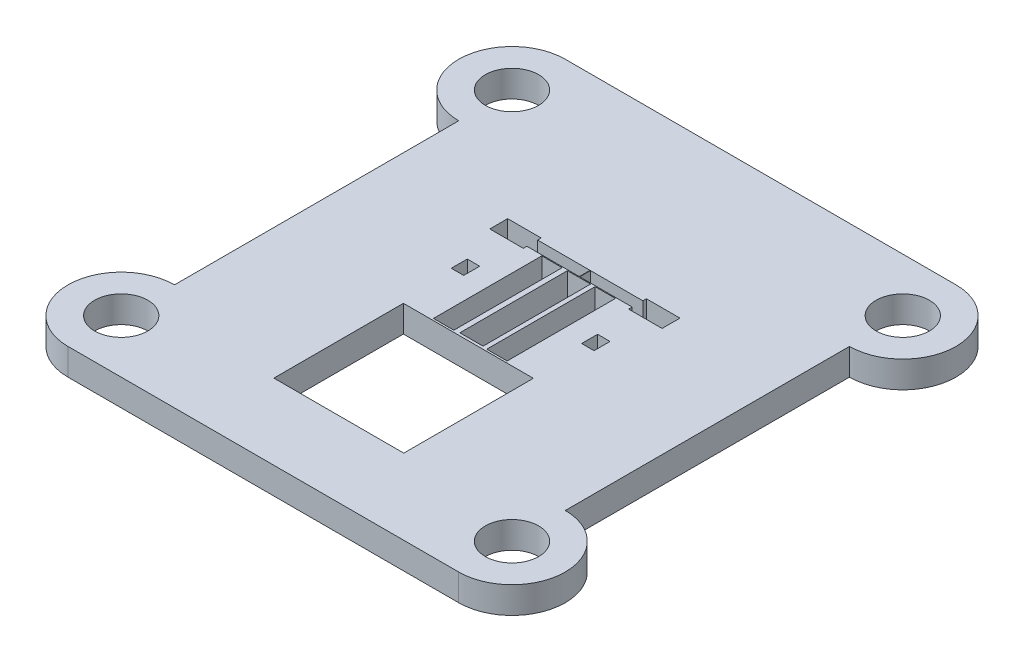
SolidWorks part; units mm, degrees
ref_plane "Front Plane" through (0, 0, 0) normal (0, 0, 1) x (1, 0, 0)
ref_plane "Top Plane" through (0, 0, 0) normal (0, 1, 0) x (1, 0, 0)
ref_plane "Right Plane" through (0, 0, 0) normal (1, 0, 0) x (0, 0, -1)
sketch "Sketch1" plane through (0, 0, 0) normal (0, 1, 0) x (1, 0, 0)
  line L0 (-110, -140) -> (80, -140)
  line L1 (80, -140) -> (80, 140)
  line L2 (80, 140) -> (-110, 140)
  line L7 (-110, -80) -> (-110, 80)
  arc A0 (-110, 140) -> (-110, 80) centre (-110, 110) ccw
  arc A1 (-110, -80) -> (-110, -140) centre (-110, -110) ccw
  circle A2 centre (-110, 110) radius 15
  circle A3 centre (-110, -110) radius 15
  dimension "D1" = 60
  dimension "D2" = 60
extrude "Boss-Extrude1" add sketch "Sketch1" along normal blind 15
ref_plane "Plane1" through (0, 0, 0) normal (0, 0, 1) x (1, 0, 0)
mirror "Mirror1" about plane through (0, 0, 0) normal (1, 0, 0) of "Boss-Extrude1"
sketch "Sketch6" plane through (0, 15, 0) normal (0, 1, 0) x (1, 0, 0)
  line L0 (-36.5722, -97.5) -> (36.5722, -97.5) construction
  line L1 (-36.5722, -97.5) -> (36.5722, -97.5)
  line L2 (-0.14, 44.06) -> (-29.63, 44.06) construction
  line L3 (-48.5, 36) -> (-29.63, 36) construction
  line L4 (-9.25, 37.5) -> (-20.75, 37.5)
  line L6 (-36.5722, -25.72) -> (-36.5722, -24.5568)
  line L7 (-36.5722, -24.5568) -> (36.5722, -24.5568)
  line L12 (-48.5, 46.06) -> (-48.5, 36) construction
  line L13 (-29.63, 46.06) -> (-48.5, 46.06) construction
  line L14 (-36.5722, -25.72) -> (-36.5722, -97.5)
  line L15 (36.5722, -25.72) -> (-36.5722, -25.72)
  line L16 (36.5722, -97.5) -> (36.5722, -25.72)
  line L17 (-36.5722, -97.5) -> (36.5722, -97.5)
  line L18 (-36.5722, -25.72) -> (-36.5722, -97.5)
  line L20 (36.5722, -97.5) -> (36.5722, -25.72)
  line L21 (-36.5722, -97.5) -> (36.5722, -97.5)
  line L22 (-0.14, 44.06) -> (-29.63, 44.06)
  line L23 (-48.5, 36) -> (-29.63, 36)
  line L24 (-48.5, 46.06) -> (-48.5, 36)
  line L25 (-29.63, 46.06) -> (-48.5, 46.06)
  line L26 (48.5, 36) -> (48.5, 46.06)
  line L27 (29.63, 36) -> (48.5, 36)
  line L28 (29.63, 38) -> (29.63, 36)
  line L29 (0.14, 38) -> (29.63, 38)
  line L30 (0.14, 44.06) -> (0.14, 38)
  line L31 (29.63, 44.06) -> (0.14, 44.06)
  line L32 (29.63, 46.06) -> (29.63, 44.06)
  line L33 (48.5, 46.06) -> (29.63, 46.06)
  line L34 (48.5, 36) -> (48.5, 46.06)
  line L35 (29.63, 36) -> (48.5, 36)
  line L36 (29.63, 38) -> (29.63, 36)
  line L37 (0.14, 38) -> (29.63, 38)
  line L38 (0.14, 44.06) -> (0.14, 38)
  line L39 (29.63, 44.06) -> (0.14, 44.06)
  line L40 (29.63, 46.06) -> (29.63, 44.06)
  line L41 (48.5, 46.06) -> (29.63, 46.06)
  line L42 (-48.5, 46.06) -> (-48.5, 36)
  line L43 (-29.63, 46.06) -> (-48.5, 46.06)
  line L44 (-29.63, 44.06) -> (-29.63, 46.06)
  line L45 (-0.14, 44.06) -> (-29.63, 44.06)
  line L46 (-0.14, 38) -> (-0.14, 44.06)
  line L47 (-29.63, 38) -> (-0.14, 38)
  line L48 (-29.63, 36) -> (-29.63, 38)
  line L49 (-48.5, 36) -> (-29.63, 36)
  line L50 (-48.5, 46.06) -> (-48.5, 36)
  line L51 (-29.63, 46.06) -> (-48.5, 46.06)
  line L52 (-29.63, 44.06) -> (-29.63, 46.06)
  line L53 (-0.14, 44.06) -> (-29.63, 44.06)
  line L54 (-0.14, 38) -> (-0.14, 44.06)
  line L55 (-29.63, 38) -> (-0.14, 38)
  line L56 (-29.63, 36) -> (-29.63, 38)
  line L57 (-48.5, 36) -> (-29.63, 36)
  line L58 (-9.25, -23.5) -> (-9.25, 37.5) construction
  line L59 (-20.75, -23.5) -> (-9.25, -23.5) construction
  line L60 (-20.75, 37.5) -> (-20.75, -23.5) construction
  line L61 (-40.19, 15) -> (-40.19, 6) construction
  line L62 (-6.31, 37.5) -> (-6.31, -23.06)
  line L63 (6.75, 37.5) -> (-6.31, 37.5)
  line L64 (6.75, -23.06) -> (6.75, 37.5)
  line L65 (-6.31, -23.06) -> (6.75, -23.06)
  line L66 (-6.31, 37.5) -> (-6.31, -23.06)
  line L67 (6.75, 37.5) -> (-6.31, 37.5)
  line L68 (6.75, -23.06) -> (6.75, 37.5)
  line L69 (-6.31, -23.06) -> (6.75, -23.06)
  line L70 (9.25, 37.5) -> (9.25, -23.5)
  line L71 (20.75, 37.5) -> (9.25, 37.5)
  line L72 (20.75, -23.5) -> (20.75, 37.5)
  line L73 (9.25, -23.5) -> (20.75, -23.5)
  line L74 (9.25, 37.5) -> (9.25, -23.5)
  line L75 (20.75, 37.5) -> (9.25, 37.5)
  line L76 (20.75, -23.5) -> (20.75, 37.5)
  line L77 (9.25, -23.5) -> (20.75, -23.5)
  line L78 (-40.19, 15) -> (-40.19, 6)
  line L79 (-33.19, 15) -> (-40.19, 15)
  line L80 (-33.19, 6) -> (-33.19, 15)
  line L81 (-40.19, 6) -> (-33.19, 6)
  line L82 (-40.19, 15) -> (-40.19, 6)
  line L83 (-33.19, 15) -> (-40.19, 15)
  line L84 (-33.19, 6) -> (-33.19, 15)
  line L85 (-40.19, 6) -> (-33.19, 6)
  line L86 (33.19, 15) -> (33.19, 6)
  line L87 (40.19, 15) -> (33.19, 15)
  line L88 (40.19, 6) -> (40.19, 15)
  line L89 (33.19, 6) -> (40.19, 6)
  line L90 (33.19, 15) -> (33.19, 6)
  line L91 (40.19, 15) -> (33.19, 15)
  line L92 (40.19, 6) -> (40.19, 15)
  line L93 (33.19, 6) -> (40.19, 6)
  line L94 (40.19, 6) -> (40.19, 15) construction
  line L95 (-9.25, -23.5) -> (-9.25, 37.5)
  line L96 (-20.75, -23.5) -> (-9.25, -23.5)
  line L97 (-20.75, 37.5) -> (-20.75, -23.5)
  line L98 (-40.19, 15) -> (-40.19, 6)
  line L99 (40.19, 6) -> (40.19, 15)
  line L100 (36.5722, -24.5568) -> (36.5722, -25.72)
  dimension "D2" = 0
  dimension "D3" = 0
  dimension "D4" = 0
  dimension "D5" = 0
  dimension "D6" = 0
  dimension "D7" = 0
  dimension "D8" = 0
extrude "Cut-Extrude1" cut sketch "Sketch6" against normal up to next
sketch "Sketch7" plane through (0, 0, 0) normal (0, -1, 0) x (1, 0, 0)
  line L0 (0, 0) -> (0, -158.586) construction
  line L1 (40.003, -88.065) -> (-75.9228, -88.065) construction
  line L2 (40.003, -113.065) -> (40.003, -63.065) construction
  line L5 (60, -114.065) -> (38, -114.065)
  line L6 (-60, -62.065) -> (-38, -62.065)
  line L7 (-60, -62.065) -> (-60, -114.065)
  line L8 (-60, -114.065) -> (-38, -114.065)
  line L9 (-38, -62.065) -> (-38, -114.065)
  line L10 (38, -62.065) -> (38, -114.065)
  line L11 (60, -62.065) -> (38, -62.065)
  line L12 (60, -62.065) -> (60, -114.065)
  dimension "D1" = 38
  dimension "D2" = 22
  dimension "D3" = 52
  dimension "D4" = 26
extrude "Cut-Extrude2" cut sketch "Sketch7" against normal blind 10
fillet "Fillet1" radius 1 16 edges at (49, 0, -62.065) (60, 0, -88.065) (49, 0, -114.065) (49, 10, -114.065) (60, 10, -88.065) (49, 10, -62.065) (38, 0, -88.065) (38, 10, -88.065) (-49, 10, -114.065) (-38, 10, -88.065) (-60, 10, -88.065) (-49, 10, -62.065) (-49, 0, -114.065) (-38, 0, -88.065) (-49, 0, -62.065) (-60, 0, -88.065)
